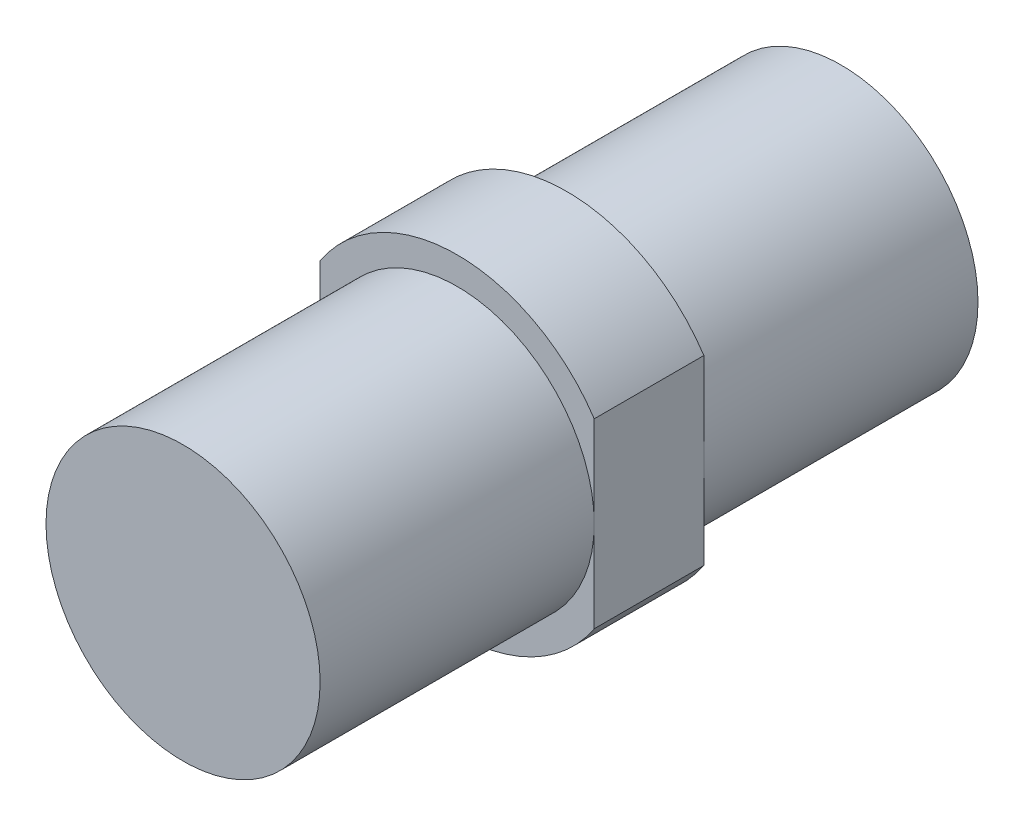
from build123d import *

# Parameters (mm, degrees)
BOSS_EXTRUDE1_DEPTH = 4
SKETCH2_W           = 5
SKETCH2_H           = 10
SKETCH3_W           = 5
SKETCH3_H           = 10


with BuildPart() as part:
    # Sketch1 → Boss-Extrude1 (new body)
    with BuildSketch(Plane.XY.offset(4)):
        with BuildLine():
            Line((5, -3.31662479), (5, 3.31662479))
            ThreePointArc((5, 3.31662479), (0, 6), (-5, 3.31662479))
            Line((-5, 3.31662479), (-5, -3.31662479))
            ThreePointArc((-5, -3.31662479), (0, -6), (5, -3.31662479))
        make_face()
    extrude(amount=-BOSS_EXTRUDE1_DEPTH)

    # Sketch2 → Revolve1 (revolve)
    with BuildSketch(Plane(origin=(0, 0, 0), x_dir=(1, 0, 0), z_dir=(0, 1, 0))):
        with Locations((2.5, -9)):
            Rectangle(SKETCH2_W, SKETCH2_H)
    revolve(axis=Axis((0, 0, 4), (0, 0, 1)))

    # Sketch3 → Revolve2 (revolve)
    with BuildSketch(Plane.XZ, mode=Mode.PRIVATE) as revolve2_sk:
        with Locations((2.5, -5)):
            Rectangle(SKETCH3_W, SKETCH3_H)
    revolve(revolve2_sk.sketch.rotate(Axis((0, 0, 0), (0, 0, -1)), 180), axis=Axis((0, 0, 0), (0, 0, -1)))


solid = part.part
